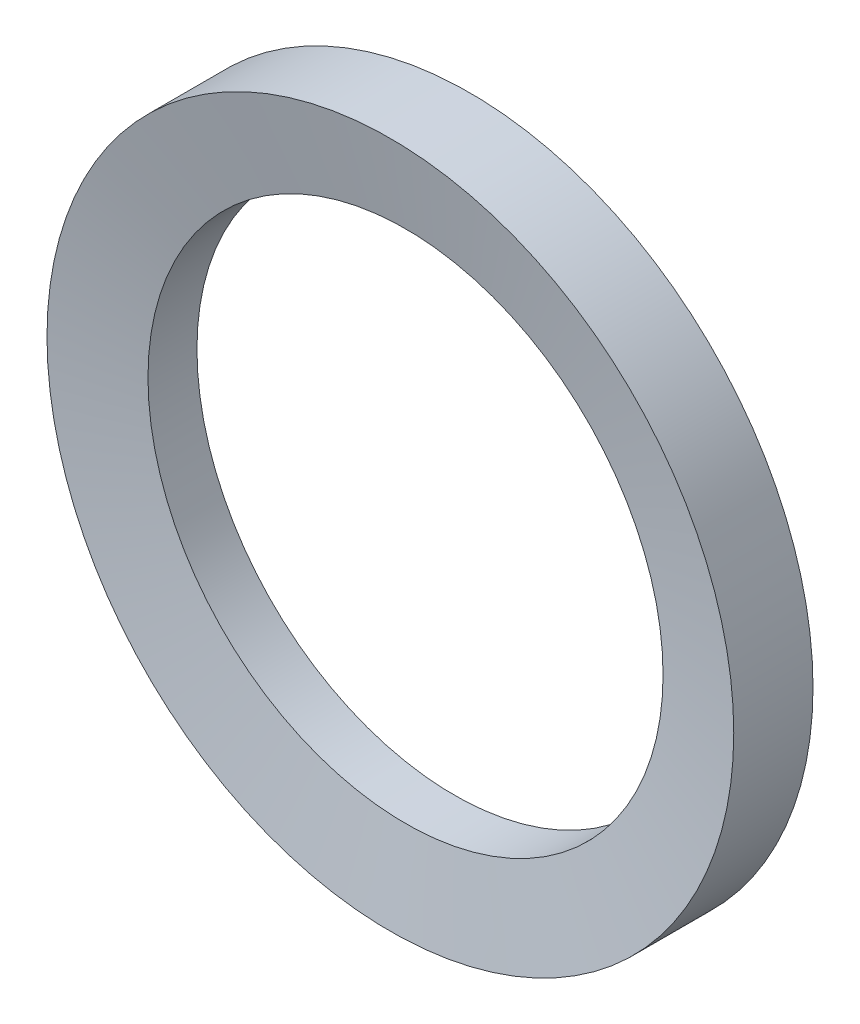
from build123d import *

# Parameters (mm, degrees)
SKETCH1_R           = 26
SKETCH1_R_2         = 19.5
BOSS_EXTRUDE1_DEPTH = 3


with BuildPart() as part:
    # Sketch1 → Boss-Extrude1 (new, symmetric)
    with BuildSketch(Plane.XY):
        Circle(SKETCH1_R)
        Circle(SKETCH1_R_2, mode=Mode.SUBTRACT)
    extrude(amount=BOSS_EXTRUDE1_DEPTH, both=True)

    # Cut-Extrude1 cone 1 section (through the dimple's axis) → Cut-Extrude1 (revolve, cut)
    with BuildSketch(Plane(origin=(0, 0, 3), x_dir=(0, -1, 0), z_dir=(1, 0, 0))):
        Polygon((0, 0), (26, 0), (0, 4.584501498), align=None)
    cut_extrude1 = revolve(axis=Axis((0, 0, 3), (0, 0, -1)), mode=Mode.SUBTRACT)

    # Mirror1: Cut-Extrude1 across plane
    add(cut_extrude1.mirror(Plane.XY), mode=Mode.SUBTRACT)


solid = part.part
